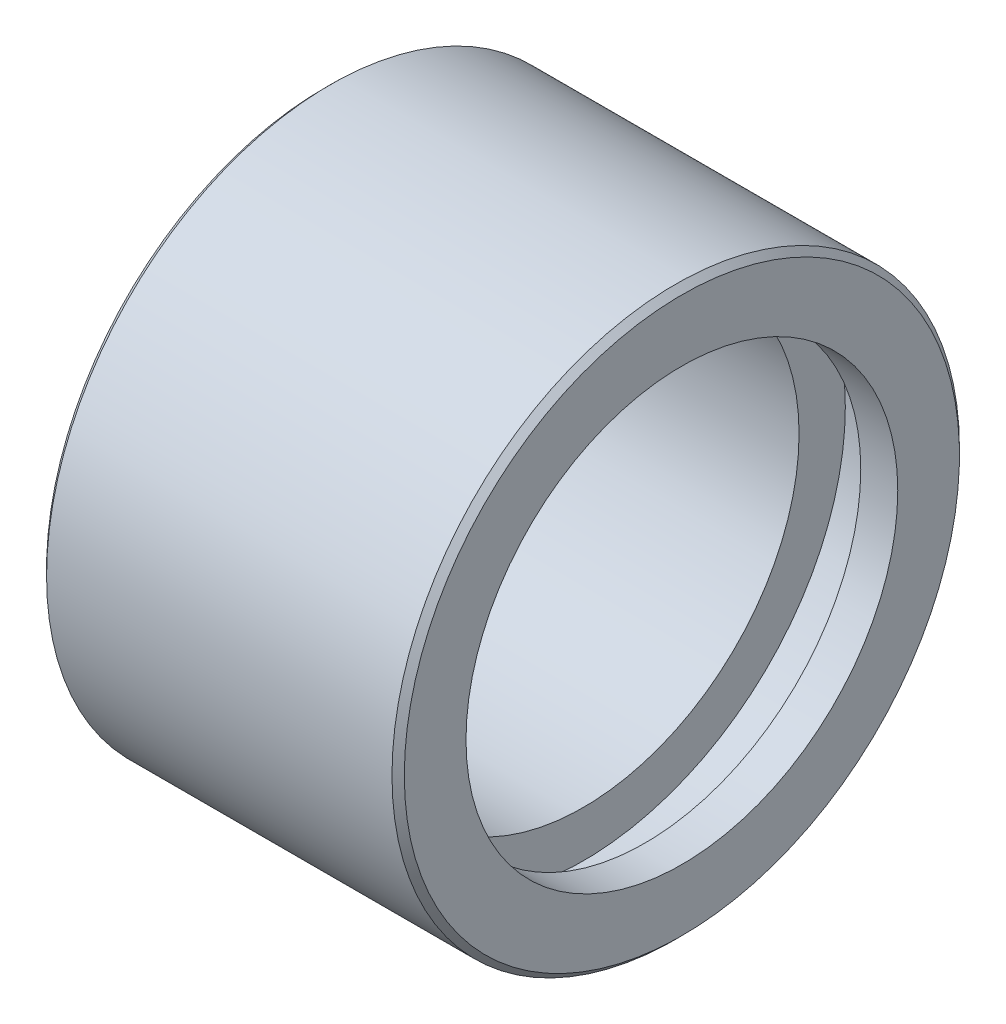
from build123d import *

# Parameters (mm, degrees)
CHAMFER_1_SIZE = 0.5


with BuildPart() as part:
    # 草图1 → 旋转1 (revolve)
    with BuildSketch(Plane.XY, mode=Mode.PRIVATE) as revolve_1_sk:
        Polygon((0, 17.5), (21, 17.5), (21, 21.25), (26, 21.25), (26, 17.5), (29, 17.5), (29, 23), (0, 23), align=None)
    revolve(revolve_1_sk.sketch.rotate(Axis((0, 0, 0), (1, 0, 0)), 90), axis=Axis((0, 0, 0), (1, 0, 0)))

    # 倒角1
    chamfer_1_edges = [part.edges().sort_by_distance(p)[0] for p in [
        (29, 0, -23),
        (0, 0, -23),
    ]]
    chamfer(chamfer_1_edges, length=CHAMFER_1_SIZE)


solid = part.part
